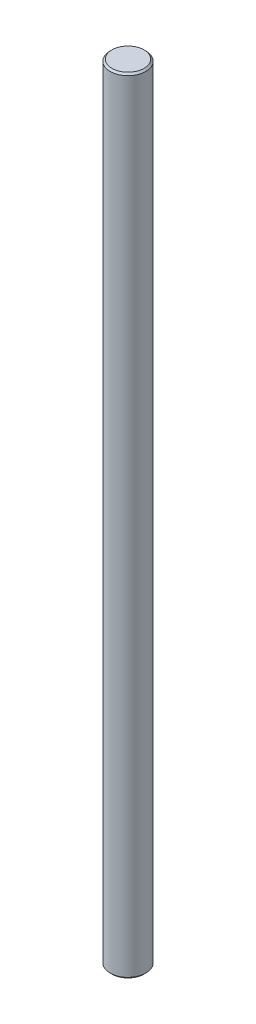
from build123d import *
from build123d.topology import SkipClean

# Parameters (mm, degrees)
SKETCH1_R           = 5
BOSS_EXTRUDE1_DEPTH = 220
CHAMFER1_SIZE       = 0.5
CUT_EXTRUDE1_DEPTH  = 12


with BuildPart() as part:
    # Sketch1 → Boss-Extrude1 (new body)
    with BuildSketch(Plane(origin=(0, 0, 0), x_dir=(1, 0, 0), z_dir=(0, 1, 0))):
        with Locations(Location((0, 0, 0), (0, 0, 270))):
            Circle(SKETCH1_R)
    extrude(amount=BOSS_EXTRUDE1_DEPTH)

    # Chamfer1
    chamfer1_edges = [part.edges().sort_by_distance(p)[0] for p in [
        (0, 0, -5),
        (0, 220, -5),
    ]]
    chamfer(chamfer1_edges, length=CHAMFER1_SIZE)

    # Sketch2 → Cut-Extrude1 (cut)
    with SkipClean():  # the faces are left unmerged after this step: merging them gives an invalid solid
        with BuildSketch(Plane(origin=(0, 0, 0), x_dir=(1, 0, 0), z_dir=(0, 1, 0))):
            with BuildLine():
                Line((-2.179449472, 4.5), (2.179449472, 4.5))
                ThreePointArc((2.179449472, 4.5), (0, 5), (-2.179449472, 4.5))
            make_face()
        extrude(amount=CUT_EXTRUDE1_DEPTH, mode=Mode.SUBTRACT)


solid = part.part
